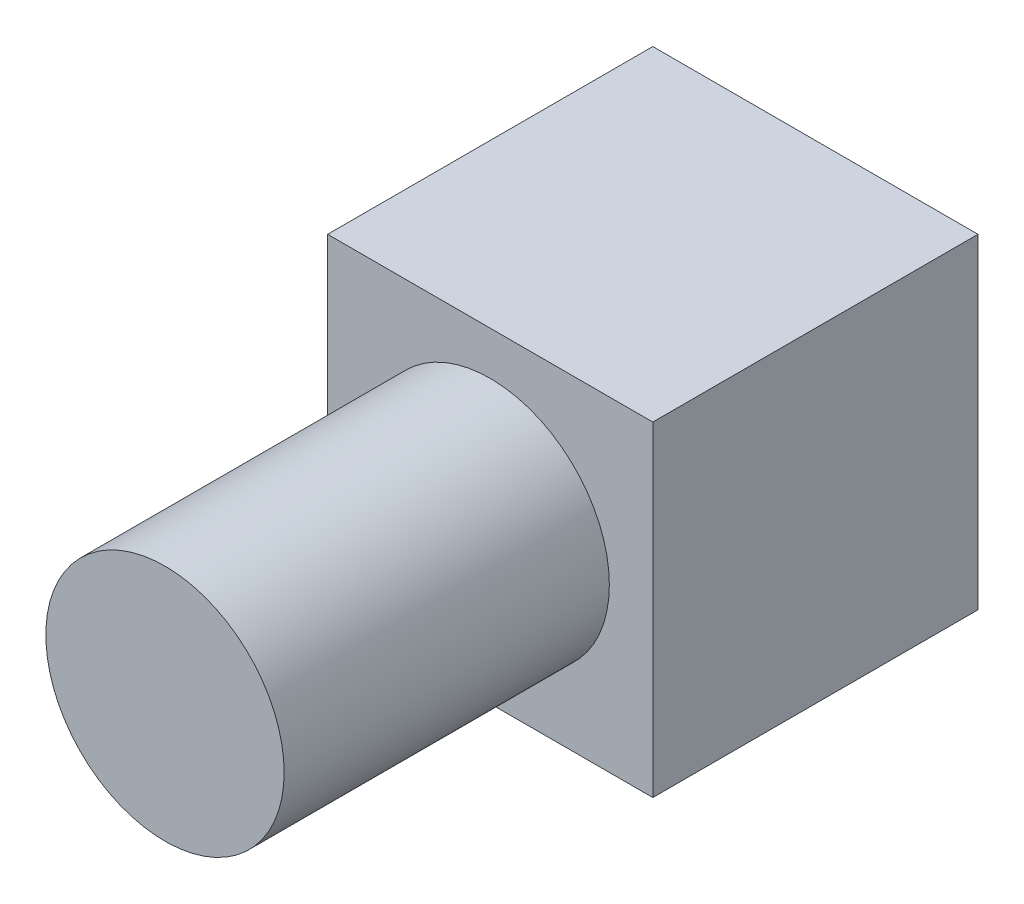
from build123d import *

# Parameters (mm, degrees)
SKETCH1_W           = 60
SKETCH1_H           = 60
BOSS_EXTRUDE1_DEPTH = 60
SKETCH2_R           = 21.984754573
BOSS_EXTRUDE2_DEPTH = 60


with BuildPart() as part:
    # Sketch1 → Boss-Extrude1 (new body)
    with BuildSketch(Plane(origin=(0, 0, 0), x_dir=(1, 0, 0), z_dir=(0, 1, 0))):
        Rectangle(SKETCH1_W, SKETCH1_H)
    extrude(amount=BOSS_EXTRUDE1_DEPTH)

    # Sketch2 → Boss-Extrude2 (add)
    with BuildSketch(Plane.XY.offset(30)):
        with Locations((0, 30)):
            Circle(SKETCH2_R)
    extrude(amount=BOSS_EXTRUDE2_DEPTH)


solid = part.part
